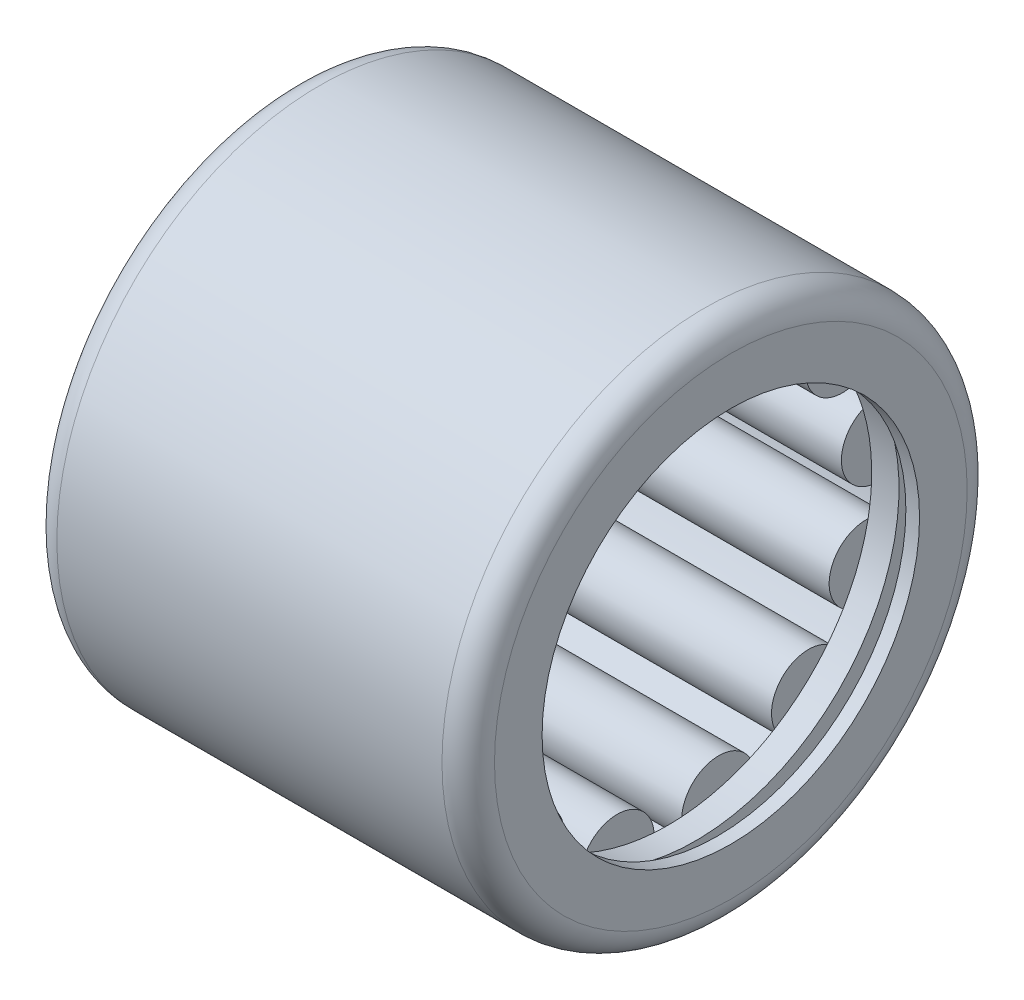
from build123d import *

# Parameters (mm, degrees)
SKETCH5_W         = 0.625
SKETCH5_H         = 0.375
SKETCH6_W         = 0.4125
SKETCH6_H         = 0.2375
CIRPATTERN3_COUNT = 13
CIRPATTERN2_COUNT = 13
FILLET1_R         = 0.6


with BuildPart() as part:
    # Sketch5 → Base-Revolve2 (revolve)
    with BuildSketch(Plane.XY, mode=Mode.PRIVATE) as base_revolve2_sk:
        with Locations((1.125, 4.84375)):
            Rectangle(SKETCH5_W, SKETCH5_H)
    base_revolve2 = revolve(base_revolve2_sk.sketch.rotate(Axis((0, 0, 0), (1, 0, 0)), 90), axis=Axis((0, 0, 0), (1, 0, 0)))

    # Sketch6 → Cut-Revolve1 (revolve, cut)
    with BuildSketch(Plane.XY):
        with Locations((1.28125, 4.725)):
            Rectangle(SKETCH6_W, SKETCH6_H)
    cut_revolve1 = revolve(axis=Axis((-4.603138189, 4.84375, 0), (1, 0, 0)), mode=Mode.SUBTRACT)

    # CirPattern3: Cut-Revolve1 ×13 about axis
    cirpattern3_axis = Axis((0, 0, 0), (1, 0, 0))
    for i in range(1, CIRPATTERN3_COUNT):
        add(cut_revolve1.rotate(cirpattern3_axis, i * 360 / CIRPATTERN3_COUNT), mode=Mode.SUBTRACT)

    # Sketch3 → Base-Revolve (revolve)
    with BuildSketch(Plane.XY, mode=Mode.PRIVATE) as base_revolve_sk:
        Polygon((1.4375, 5.6885), (8.5625, 5.6885), (8.5625, 5.03125), (8.875, 5.03125), (8.875, 4.84375), (1.125, 4.84375), (1.125, 5.03125), (1.4375, 5.03125), align=None)
    base_revolve = revolve(base_revolve_sk.sketch.rotate(Axis((-4.603138189, 4.84375, 0), (1, 0, 0)), 90), axis=Axis((-4.603138189, 4.84375, 0), (1, 0, 0)))

    # Sketch2 → Boss-Revolve2 (revolve)
    with BuildSketch(Plane.XY, mode=Mode.PRIVATE) as boss_revolve2_sk:
        Polygon((9.6875, 4.3125), (10, 4.3125), (10, 6), (0, 6), (0, 4.3125), (0.3125, 4.3125), (0.3125, 5.6875), (9.6875, 5.6875), align=None)
    revolve(boss_revolve2_sk.sketch.rotate(Axis((0, 0, 0), (1, 0, 0)), 90), axis=Axis((0, 0, 0), (1, 0, 0)))

    # Mirror1: Base-Revolve2 across plane
    add(base_revolve2.mirror(Plane.ZY.offset(-5)))

    # CirPattern2: Base-Revolve ×13 about axis
    cirpattern2_axis = Axis((0, 0, 0), (1, 0, 0))
    for i in range(1, CIRPATTERN2_COUNT):
        add(base_revolve.rotate(cirpattern2_axis, i * 360 / CIRPATTERN2_COUNT))

    # Fillet1
    fillet1_edges = [part.edges().sort_by_distance(p)[0] for p in [
        (0, 0, -6),
        (10, 0, -6),
    ]]
    fillet(fillet1_edges, radius=FILLET1_R)

    # Mirror2: Base-Revolve across plane
    add(base_revolve.mirror(Plane.ZY.offset(-5)))


solid = part.part
